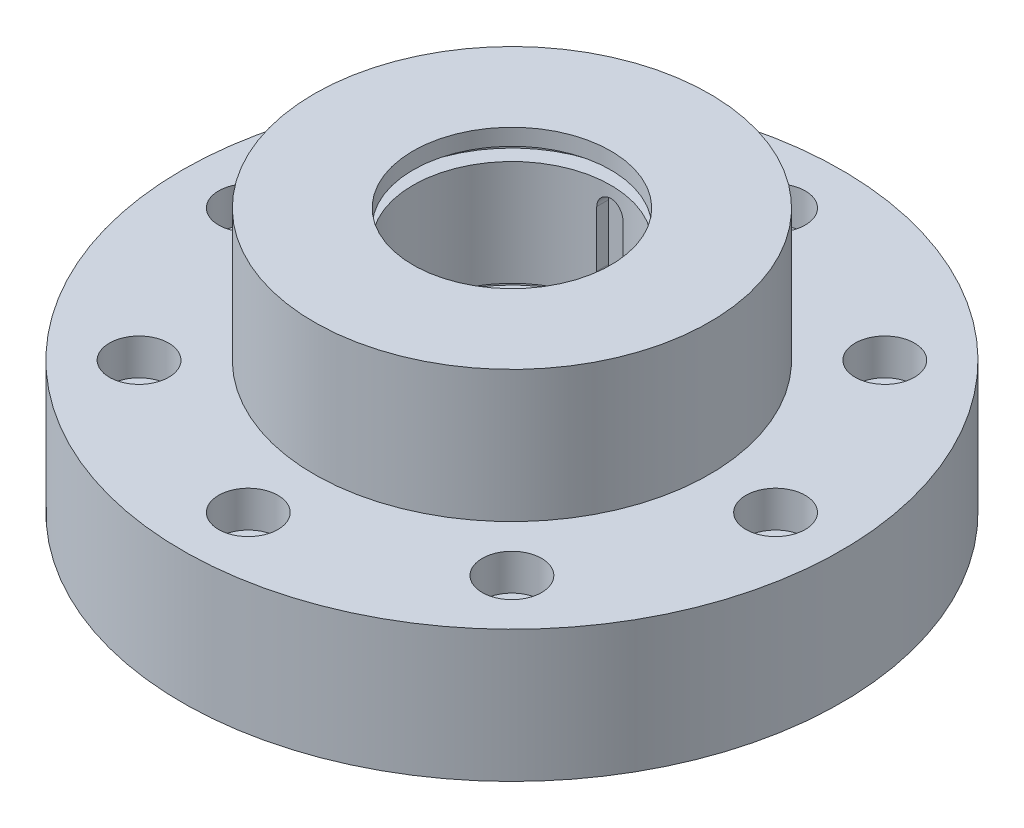
from build123d import *

# Parameters (mm, degrees)
SKETCH_2_R          = 9
CUT_EXTRUDE_1_DEPTH = 11
CUT_EXTRUDE_2_REACH = 152.336
SKETCH_3_R          = 5.25
CUT_EXTRUDE_START   = -7.5
SKETCH_6_W          = 8
SKETCH_6_H          = 7
CUT_EXTRUDE_3_DEPTH = 17
CUT_EXTRUDE_4_DEPTH = 7


with BuildPart() as part:
    # 草图1 → 旋转1 (revolve)
    with BuildSketch(Plane.XY, mode=Mode.PRIVATE) as revolve_1_sk:
        Polygon((30, 64.090909091), (60, 64.090909091), (60, 24.090909091), (100, 24.090909091), (100, -15.909090909), (57.5, -15.909090909), (57.5, -35.909090909), (40, -35.909090909), (40, -5.909090909), (35, -5.909090909), (35, 14.090909091), (30, 14.090909091), (30, 19.090909091), (35, 19.090909091), (35, 23.090909091), (30, 23.090909091), (30, 55.090909091), (35, 55.090909091), (35, 59.090909091), (30, 59.090909091), align=None)
    revolve(revolve_1_sk.sketch.rotate(Axis((0, 82.636363636, 0), (0, -1, 0)), 180), axis=Axis((0, 82.636363636, 0), (0, -1, 0)))

    # 草图2 → 切除-拉伸1 (cut)
    with BuildSketch(Plane(origin=(0, 24.090909091, 0), x_dir=(1, 0, 0), z_dir=(0, 1, 0))):
        with Locations(Location((80, 0, 0), (0, 0, 180))):
            Circle(SKETCH_2_R)
        with Locations(Location((56.568542495, -56.568542495, 0), (0, 0, 180))):
            Circle(SKETCH_2_R)
        with Locations(Location((0, -80, 0), (0, 0, 180))):
            Circle(SKETCH_2_R)
        with Locations(Location((-56.568542495, -56.568542495, 0), (0, 0, 180))):
            Circle(SKETCH_2_R)
        with Locations(Location((-80, 0, 0), (0, 0, 180))):
            Circle(SKETCH_2_R)
        with Locations(Location((-56.568542495, 56.568542495, 0), (0, 0, 180))):
            Circle(SKETCH_2_R)
        with Locations(Location((0, 80, 0), (0, 0, 180))):
            Circle(SKETCH_2_R)
        with Locations(Location((56.568542495, 56.568542495, 0), (0, 0, 180))):
            Circle(SKETCH_2_R)
    extrude(amount=-CUT_EXTRUDE_1_DEPTH, mode=Mode.SUBTRACT)

    # 草图3 → 切除-拉伸2 (cut, up to next)
    with BuildSketch(Plane(origin=(0, 13.090909091, 0), x_dir=(1, 0, 0), z_dir=(0, 1, 0)), mode=Mode.PRIVATE) as cut_extrude_2_sk1:
        with Locations(Location((56.568542495, 56.568542495, 0), (0, 0, 180))):
            Circle(SKETCH_3_R)
    cut_extrude_2_tool1 = extrude(cut_extrude_2_sk1.sketch, amount=-CUT_EXTRUDE_2_REACH, mode=Mode.PRIVATE) & part.part
    # 草图3 → 切除-拉伸2 (cut, up to next)
    with BuildSketch(Plane(origin=(0, 13.090909091, 0), x_dir=(1, 0, 0), z_dir=(0, 1, 0)), mode=Mode.PRIVATE) as cut_extrude_2_sk2:
        with Locations(Location((80, 0, 0), (0, 0, 180))):
            Circle(SKETCH_3_R)
    cut_extrude_2_tool2 = extrude(cut_extrude_2_sk2.sketch, amount=-CUT_EXTRUDE_2_REACH, mode=Mode.PRIVATE) & part.part
    # 草图3 → 切除-拉伸2 (cut, up to next)
    with BuildSketch(Plane(origin=(0, 13.090909091, 0), x_dir=(1, 0, 0), z_dir=(0, 1, 0)), mode=Mode.PRIVATE) as cut_extrude_2_sk3:
        with Locations(Location((56.568542495, -56.568542495, 0), (0, 0, 180))):
            Circle(SKETCH_3_R)
    cut_extrude_2_tool3 = extrude(cut_extrude_2_sk3.sketch, amount=-CUT_EXTRUDE_2_REACH, mode=Mode.PRIVATE) & part.part
    # 草图3 → 切除-拉伸2 (cut, up to next)
    with BuildSketch(Plane(origin=(0, 13.090909091, 0), x_dir=(1, 0, 0), z_dir=(0, 1, 0)), mode=Mode.PRIVATE) as cut_extrude_2_sk4:
        with Locations(Location((0, -80, 0), (0, 0, 180))):
            Circle(SKETCH_3_R)
    cut_extrude_2_tool4 = extrude(cut_extrude_2_sk4.sketch, amount=-CUT_EXTRUDE_2_REACH, mode=Mode.PRIVATE) & part.part
    # 草图3 → 切除-拉伸2 (cut, up to next)
    with BuildSketch(Plane(origin=(0, 13.090909091, 0), x_dir=(1, 0, 0), z_dir=(0, 1, 0)), mode=Mode.PRIVATE) as cut_extrude_2_sk5:
        with Locations(Location((-56.568542495, -56.568542495, 0), (0, 0, 180))):
            Circle(SKETCH_3_R)
    cut_extrude_2_tool5 = extrude(cut_extrude_2_sk5.sketch, amount=-CUT_EXTRUDE_2_REACH, mode=Mode.PRIVATE) & part.part
    # 草图3 → 切除-拉伸2 (cut, up to next)
    with BuildSketch(Plane(origin=(0, 13.090909091, 0), x_dir=(1, 0, 0), z_dir=(0, 1, 0)), mode=Mode.PRIVATE) as cut_extrude_2_sk6:
        with Locations(Location((-80, 0, 0), (0, 0, 180))):
            Circle(SKETCH_3_R)
    cut_extrude_2_tool6 = extrude(cut_extrude_2_sk6.sketch, amount=-CUT_EXTRUDE_2_REACH, mode=Mode.PRIVATE) & part.part
    # 草图3 → 切除-拉伸2 (cut, up to next)
    with BuildSketch(Plane(origin=(0, 13.090909091, 0), x_dir=(1, 0, 0), z_dir=(0, 1, 0)), mode=Mode.PRIVATE) as cut_extrude_2_sk7:
        with Locations(Location((-56.568542495, 56.568542495, 0), (0, 0, 180))):
            Circle(SKETCH_3_R)
    cut_extrude_2_tool7 = extrude(cut_extrude_2_sk7.sketch, amount=-CUT_EXTRUDE_2_REACH, mode=Mode.PRIVATE) & part.part
    # 草图3 → 切除-拉伸2 (cut, up to next)
    with BuildSketch(Plane(origin=(0, 13.090909091, 0), x_dir=(1, 0, 0), z_dir=(0, 1, 0)), mode=Mode.PRIVATE) as cut_extrude_2_sk8:
        with Locations(Location((0, 80, 0), (0, 0, 180))):
            Circle(SKETCH_3_R)
    cut_extrude_2_tool8 = extrude(cut_extrude_2_sk8.sketch, amount=-CUT_EXTRUDE_2_REACH, mode=Mode.PRIVATE) & part.part
    add(cut_extrude_2_tool1.solids().sort_by_distance((56.568542, 13.090909, -56.568542))[0], mode=Mode.SUBTRACT)
    add(cut_extrude_2_tool2.solids().sort_by_distance((80, 13.090909, 0))[0], mode=Mode.SUBTRACT)
    add(cut_extrude_2_tool3.solids().sort_by_distance((56.568542, 13.090909, 56.568542))[0], mode=Mode.SUBTRACT)
    add(cut_extrude_2_tool4.solids().sort_by_distance((0, 13.090909, 80))[0], mode=Mode.SUBTRACT)
    add(cut_extrude_2_tool5.solids().sort_by_distance((-56.568542, 13.090909, 56.568542))[0], mode=Mode.SUBTRACT)
    add(cut_extrude_2_tool6.solids().sort_by_distance((-80, 13.090909, 0))[0], mode=Mode.SUBTRACT)
    add(cut_extrude_2_tool7.solids().sort_by_distance((-56.568542, 13.090909, -56.568542))[0], mode=Mode.SUBTRACT)
    add(cut_extrude_2_tool8.solids().sort_by_distance((0, 13.090909, -80))[0], mode=Mode.SUBTRACT)

    # 草图5 → 切除-旋转1 (revolve, cut)
    with BuildSketch(Plane(origin=(0, 0, 0), x_dir=(0, -1, 0), z_dir=(0.9238795325112864, 0, 0.38268343236509056)), mode=Mode.PRIVATE) as cut_revolve_1_sk:
        Polygon((-4.090909091, 100), (5.909090909, 100), (0.850173924, 84.430254481), (0.850173924, 3.622054485), (-4.090909091, 3.622054485), align=None)
    revolve(cut_revolve_1_sk.sketch.rotate(Axis((47.039156362, 4.090909091, -113.562569252), (-0.3826834323650906, 0, 0.9238795325112864)), 270), axis=Axis((47.039156362, 4.090909091, -113.562569252), (-0.3826834323650906, 0, 0.9238795325112864)), mode=Mode.SUBTRACT)

    # 草图6 → 切除-拉伸3 (cut)
    with BuildSketch(Plane(origin=(0, 55.090909091, 0), x_dir=(1, 0, 0), z_dir=(0, 1, 0)).offset(CUT_EXTRUDE_START)):
        with Locations((0, 29.732137495)):
            Rectangle(SKETCH_6_W, SKETCH_6_H)
    extrude(amount=-CUT_EXTRUDE_3_DEPTH, mode=Mode.SUBTRACT)

    # 草图7 → 切除-拉伸4 (cut)
    with BuildSketch(Plane.XY.offset(-33.232137495)):
        with BuildLine():
            ThreePointArc((-4, 47.590909091), (0, 51.590909091), (4, 47.590909091))
            Line((4, 47.590909091), (-4, 47.590909091))
        make_face()
        with BuildLine():
            ThreePointArc((-4, 30.590909091), (0, 26.590909091), (4, 30.590909091))
            Line((4, 30.590909091), (-4, 30.590909091))
        make_face()
    extrude(amount=CUT_EXTRUDE_4_DEPTH, mode=Mode.SUBTRACT)


solid = part.part
